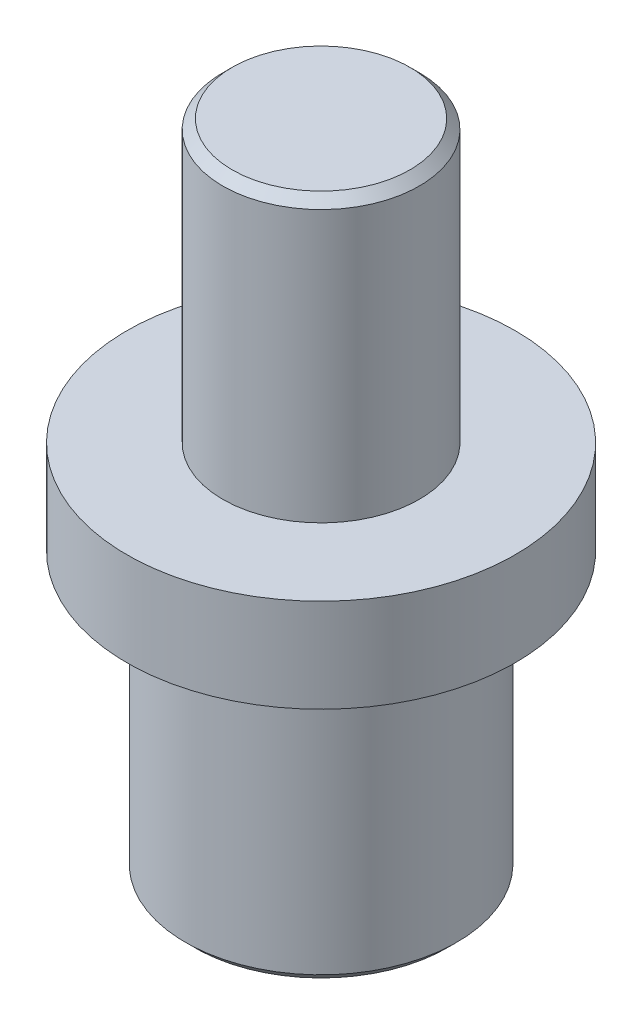
from build123d import *

# Parameters (mm, degrees)
CHAMFER1_SIZE = 0.2


with BuildPart() as part:
    # Sketch1 → Revolve1 (revolve)
    with BuildSketch(Plane.XY, mode=Mode.PRIVATE) as revolve1_sk:
        Polygon((0, 0), (0, 14), (2.1, 14), (2.1, 8), (4.15, 8), (4.15, 6), (2.9, 6), (2.9, 0), align=None)
    revolve(revolve1_sk.sketch.rotate(Axis((0, 0, 0), (0, 1, 0)), 90), axis=Axis((0, 0, 0), (0, 1, 0)))

    # Chamfer1
    chamfer1_edges = [part.edges().sort_by_distance(p)[0] for p in [
        (0, 14, 2.1),
        (0, 0, 2.9),
    ]]
    chamfer(chamfer1_edges, length=CHAMFER1_SIZE)


solid = part.part
